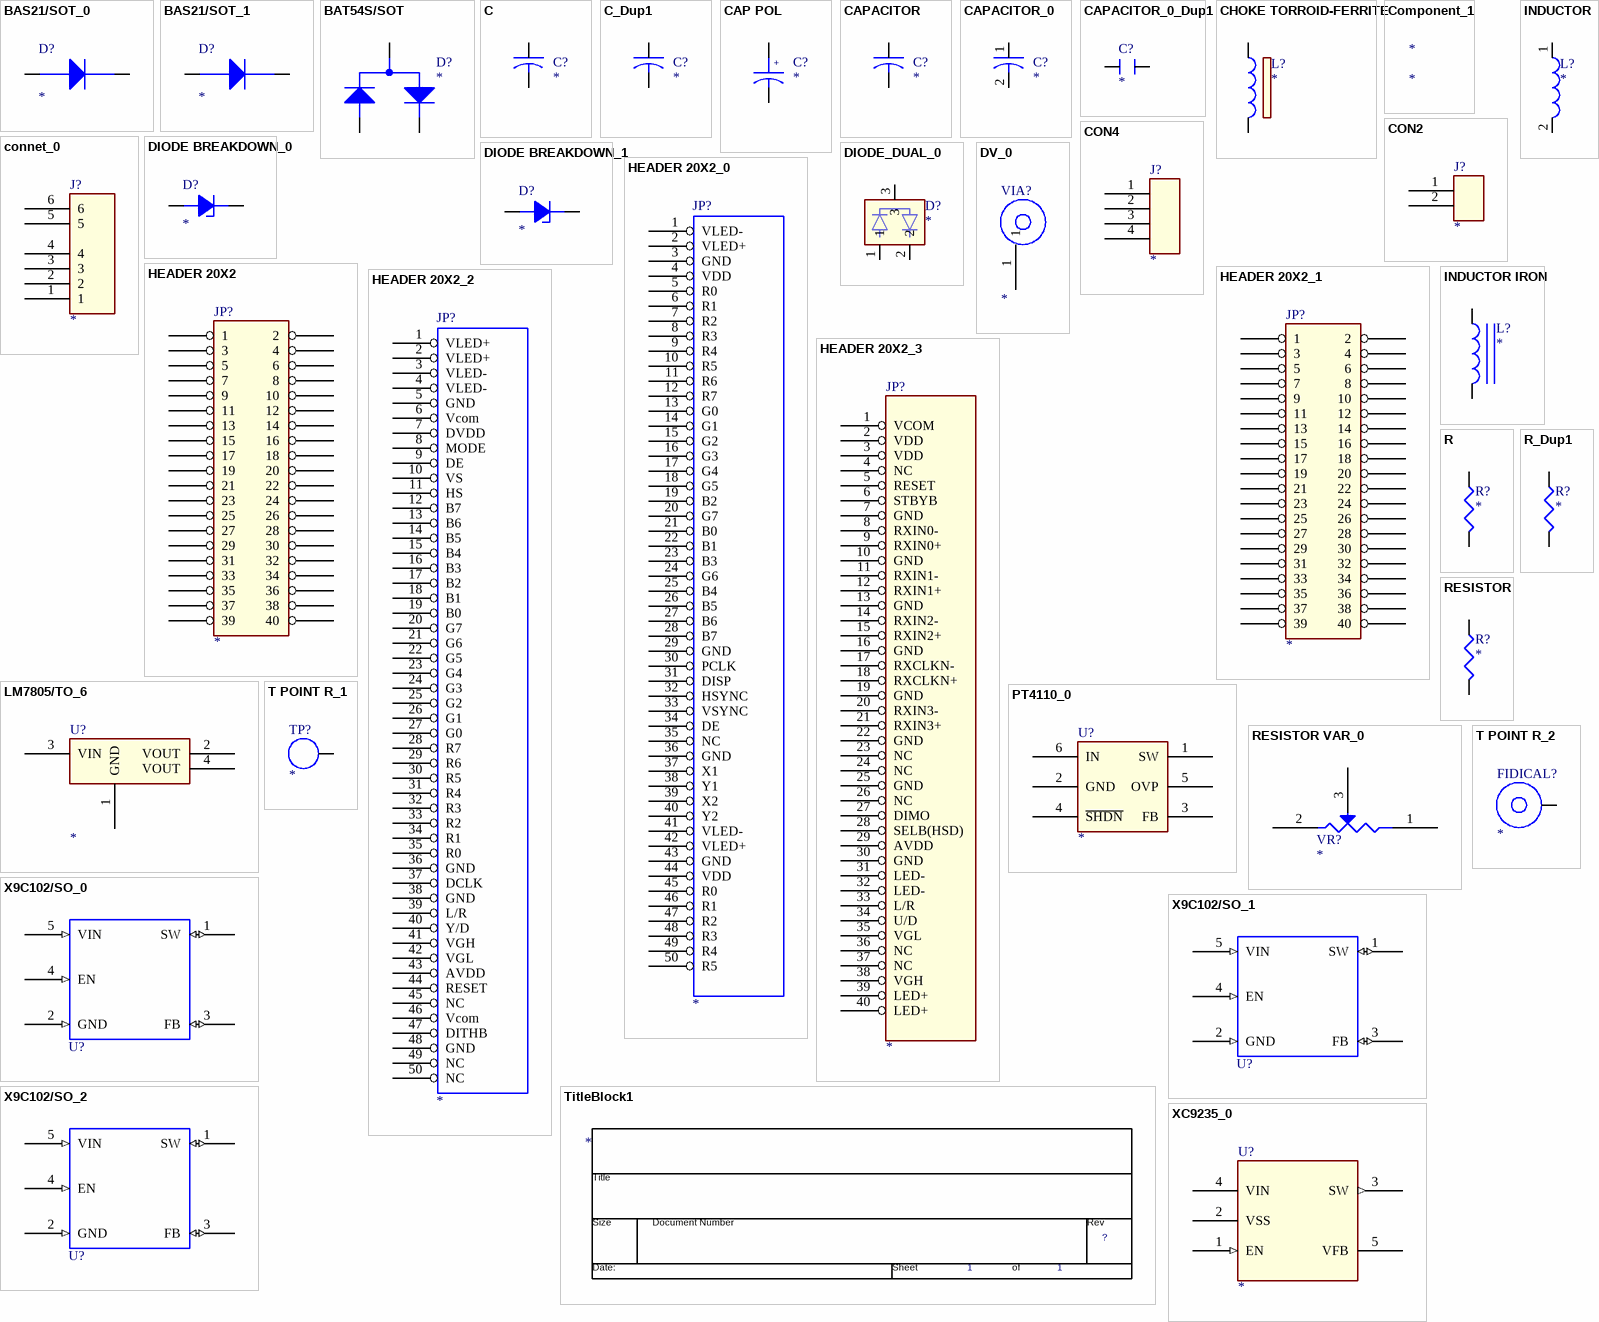
[diagram p0: symbols BAS21/SOT_0 to XC9235_0]
# Altium schematic symbol library MISC82162-5.SchLib: 38 symbols
Pins are listed as number, name and electrical type; pins without a type are passive.


## BAS21/SOT_0
designator D?
pins: 1 CATHODE, 2 ANODE

## BAS21/SOT_1
designator D?
pins: 1 ANODE, 2 CATHODE

## BAT54S/SOT
designator D?
pins: 1, 2, 3

## C
designator C?
footprint C0402
pins: 1, 2

## C_Dup1
designator C?
pins: 1, 2

## CAP POL
designator C?
pins: 1, 2

## CAPACITOR
designator C?
pins: 1, 2

## CAPACITOR_0
designator C?
pins: 1, 2

## CAPACITOR_0_Dup1
designator C?
pins: 1, 2

## CHOKE TORROID-FERRITE
designator L?
pins: 1, 2

## Component_1
designator *

## CON2
designator J?
pins: 1, 2

## CON4
designator J?
pins: 1, 2, 3, 4

## connet_0
designator J?
pins: 1, 2, 3, 4, 5, 6

## DIODE BREAKDOWN_0
designator D?
pins: 1 CATHODE, 2 ANODE

## DIODE BREAKDOWN_1
designator D?
pins: 1 ANODE, 2 CATHODE

## DIODE_DUAL_0
designator D?
pins: 1, 2, 3

## DV_0
designator VIA?
pins: 1

## HEADER 20X2
designator JP?
pins: 1, 2, 3, 4, 5, 6, 7, 8, 9, 10, 11, 12, 13, 14, 15, 16, 17, 18, 19, 20, 21, 22, 23, 24, 25, 26, 27, 28, 29, 30, 31, 32, 33, 34, 35, 36, 37, 38, 39, 40

## HEADER 20X2_0
designator JP?
pins: 1 VLED-, 2 VLED+, 3 GND, 4 VDD, 5 R0, 6 R1, 7 R2, 8 R3, 9 R4, 10 R5, 11 R6, 12 R7, 13 G0, 14 G1, 15 G2, 16 G3, 17 G4, 18 G5, 19 B2, 20 G7, 21 B0, 22 B1, 23 B3, 24 G6, 25 B4, 26 B5, 27 B6, 28 B7, 29 GND, 30 PCLK, 31 DISP, 32 HSYNC, 33 VSYNC, 34 DE, 35 NC, 36 GND, 37 X1, 38 Y1, 39 X2, 40 Y2, 41 VLED-, 42 VLED+, 43 GND, 44 VDD, 45 R0, 46 R1, 47 R2, 48 R3, 49 R4, 50 R5

## HEADER 20X2_1
designator JP?
pins: 1, 2, 3, 4, 5, 6, 7, 8, 9, 10, 11, 12, 13, 14, 15, 16, 17, 18, 19, 20, 21, 22, 23, 24, 25, 26, 27, 28, 29, 30, 31, 32, 33, 34, 35, 36, 37, 38, 39, 40

## HEADER 20X2_2
designator JP?
pins: 1 VLED+, 2 VLED+, 3 VLED-, 4 VLED-, 5 GND, 6 Vcom, 7 DVDD, 8 MODE, 9 DE, 10 VS, 11 HS, 12 B7, 13 B6, 14 B5, 15 B4, 16 B3, 17 B2, 18 B1, 19 B0, 20 G7, 21 G6, 22 G5, 23 G4, 24 G3, 25 G2, 26 G1, 27 G0, 28 R7, 29 R6, 30 R5, 31 R4, 32 R3, 33 R2, 34 R1, 35 R0, 36 GND, 37 DCLK, 38 GND, 39 L/R, 40 Y/D, 41 VGH, 42 VGL, 43 AVDD, 44 RESET, 45 NC, 46 Vcom, 47 DITHB, 48 GND, 49 NC, 50 NC

## HEADER 20X2_3
designator JP?
pins: 1 VCOM, 2 VDD, 3 VDD, 4 NC, 5 RESET, 6 STBYB, 7 GND, 8 RXIN0-, 9 RXIN0+, 10 GND, 11 RXIN1-, 12 RXIN1+, 13 GND, 14 RXIN2-, 15 RXIN2+, 16 GND, 17 RXCLKN-, 18 RXCLKN+, 19 GND, 20 RXIN3-, 21 RXIN3+, 22 GND, 23 NC, 24 NC, 25 GND, 26 NC, 27 DIMO, 28 SELB(HSD), 29 AVDD, 30 GND, 31 LED-, 32 LED-, 33 L/R, 34 U/D, 35 VGL, 36 NC, 37 NC, 38 VGH, 39 LED+, 40 LED+

## INDUCTOR
designator L?
pins: 1, 2

## INDUCTOR IRON
designator L?
pins: 1, 2

## LM7805/TO_6
designator U?
pins: 1 GND (power), 2 VOUT, 3 VIN, 4 VOUT

## PT4110_0
designator U?
footprint SOT89-5
pins: 1 SW, 2 GND, 3 FB, 4 ~{SHDN}, 5 OVP, 6 IN

## R
designator R?
pins: 1, 2

## R_Dup1
designator R?
pins: 1, 2

## RESISTOR
designator R?
pins: 1, 2

## RESISTOR VAR_0
designator VR?
pins: 1, 2, 3

## T POINT R_1
designator TP?
pins: 1 TP

## T POINT R_2
designator FIDICAL?
footprint FIDICALMARK
pins: 1 TP

## TitleBlock1
designator *  Page Count: 1  (graphical)

## X9C102/SO_0
designator U?
pins: 1 SW (io), 2 GND (in), 3 FB (io), 4 EN (in), 5 VIN (in)

## X9C102/SO_1
designator U?
pins: 1 SW (io), 2 GND (in), 3 FB (io), 4 EN (in), 5 VIN (in), 6 VCC (power) hidden to VCC

## X9C102/SO_2
designator U?
pins: 1 SW (io), 2 GND (in), 3 FB (io), 4 EN (in), 5 VIN (in)

## XC9235_0
designator U?
pins: 1 EN (in), 2 VSS (power), 3 SW (out), 4 VIN (power), 5 VFB (power)